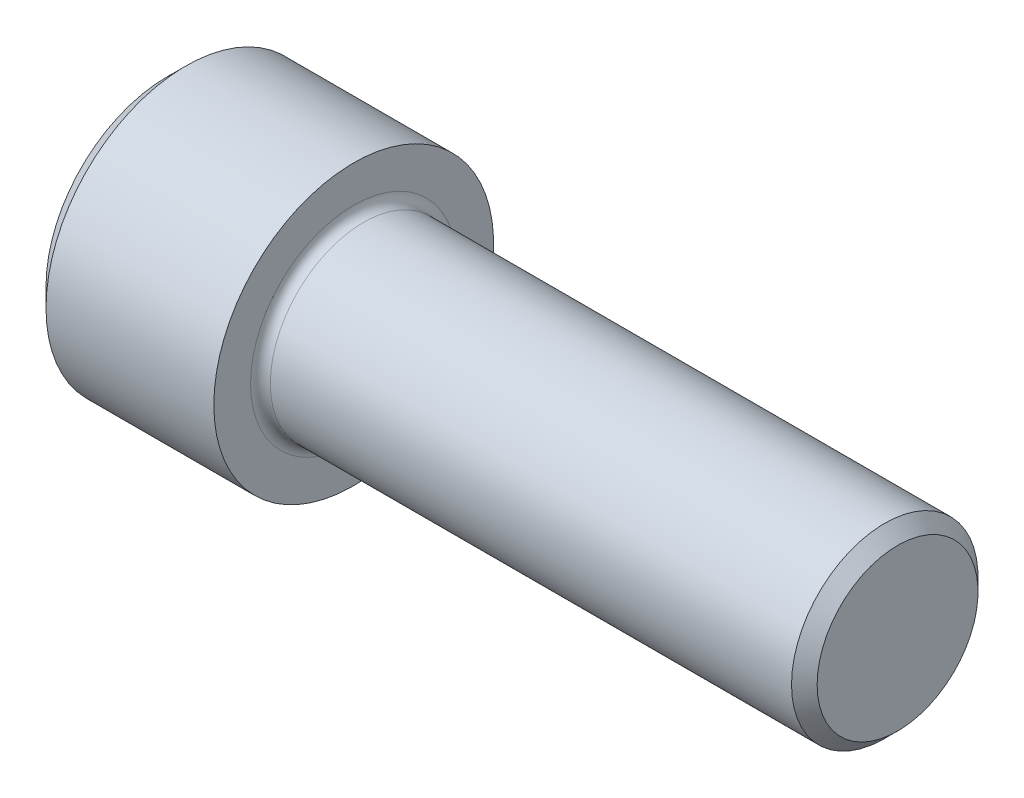
SolidWorks part; units mm, degrees
revolve "Base-Revolve" add sketch "BodySke"
sketch "BodySke" plane through (0, 0, 0) normal (0, 0, 1) x (1, 0, 0)
  line L0 (0, 0) -> (0, 15.6)
  line L1 (2.4, 18) -> (24, 18)
  line L2 (24, 18) -> (24, 12)
  line L3 (24, 12) -> (92.352, 12)
  line L4 (94, 10.352) -> (94, 0)
  line L5 (94, 0) -> (0, 0)
  line L6 (-31.75, 0) -> (127, 0) construction
  line L7 (0, 15.6) -> (2.4, 18)
  line L8 (94, 10.352) -> (92.352, 12)
  line L9 (0, -15.6) -> (2.4, -18) construction
  line L10 (94, -10.352) -> (92.352, -12) construction
  line L11 (27, 9.525) -> (27, 3.175) construction
  line L12 (44, 9.525) -> (44, 3.175) construction
  line L13 (44, 9.525) -> (44, 3.175) construction
  dimension "Diameter" = 24
  dimension "Head_ht" = 24
  dimension "Length" = 70
  dimension "Body_ch_ang" = 45
  dimension "Head_dia" = 36
  dimension "Head_ch_ang" = 45
  dimension "Minor_dia" = 20.704
  dimension "Advance" = 3
  dimension "Thread_nom" = 50
  dimension "Thread_length" = 50
  dimension "Head_ch_ht" = 2.4
cosmetic thread "ThreadCosmetic" [suppressed]
fillet "Fillet1" radius 1.27 1 edges at (24, 0, 12)
ref_plane "Plane1" through (0, 0, 0) normal (0, 0, 1) x (1, 0, 0)
ref_plane "Plane2" through (0, 0, 0) normal (0, 1, 0) x (1, 0, 0)
ref_plane "Plane3" through (0, 0, 0) normal (1, 0, 0) x (0, 0, -1)
other "Configuration Table"
sketch "Sketch2" plane through (0, 0, 0) normal (0, 0, 1) x (1, 0, 0)
  line L0 (0, 9.5) -> (12, 9.5)
  line L1 (12, 9.5) -> (17.4848, 0)
  line L2 (-31.75, 0) -> (127, 0) construction
  line L3 (17.4848, 0) -> (0, 0)
  line L4 (0, 0) -> (0, 9.5)
  line L5 (0, 15.6) -> (0, -15.6) construction
  line L6 (0, 0) -> (47.625, 0) construction
  line L7 (24, -18) -> (24, 18) construction
revolve "Hex-PreBroach" cut sketch "Sketch2" angle 360 about L6
sketch "Sketch3" plane through (0, 0, 0) normal (-1, 0, 0) x (0, 0.5, 0.866)
  line L0 (5.4848, 9.5) -> (-5.4848, 9.5)
  line L1 (-5.4848, 9.5) -> (-10.9697, 0)
  line L2 (5.4848, 9.5) -> (10.9697, 0)
  line L3 (5.4848, -9.5) -> (10.9697, 0)
  line L4 (5.4848, -9.5) -> (-5.4848, -9.5)
  line L5 (-5.4848, -9.5) -> (-10.9697, 0)
extrude "Hex" cut sketch "Sketch3" against normal blind 12
sketch "Sketch4" plane through (0, 0, 0) normal (-1, 0, 0) x (0, 0, 1)
  line L0 (0, 0) -> (10.1727, 0)
  line L1 (0, 0) -> (6.1484, 3.5498) construction
  line L2 (0, 0) -> (5.0863, 8.8098)
  line L3 (8.4417, 2.1022) -> (9.7612, 2.864)
  line L4 (6.0414, 6.2596) -> (7.3609, 7.0215)
  arc A0 (8.4417, 2.1022) -> (6.0414, 6.2596) centre (0, 0) ccw
  arc A1 (10.1727, 0) -> (9.7612, 2.864) centre (0, 0) ccw
  arc A2 (5.0863, 8.8098) -> (7.3609, 7.0215) centre (0, 0) cw
extrude "Spline" [suppressed] cut sketch "Sketch4" against normal blind 12.573
pattern_circular "CirPattern1" [suppressed] count 6 every 60
sketch "Sketch5" plane through (0, 0, 0) normal (0, 0, 1) x (1, 0, 0)
  line L0 (-31.75, 0) -> (127, 0) construction
  line L2 (0, 15.6) -> (0, -15.6) construction
  circle A0 centre (7.3, 0) radius 1.075
  dimension "Drilled_hole_dia" = 2.15
  dimension "Drilled_hole_loc" = 7.3
extrude "Hole" [suppressed] cut sketch "Sketch5" against normal through all and the other way through all
pattern_circular "Drilled-4" [suppressed] count 2 every 60
pattern_circular "Drilled-6" [suppressed] count 3 every 60
sketch "ThdSchSke" plane through (0, 0, 0) normal (0, 0, 1) x (1, 0, 0)
  line L0 (44, -10.352) -> (42.8461, -12)
  line L1 (44, -10.352) -> (45.1539, -12)
  line L2 (45.1539, -12) -> (45.1539, -15)
  line L3 (-3.175, 0) -> (5.1513, 0) construction
  line L5 (45.1539, -15) -> (42.8461, -15)
  line L6 (42.8461, -15) -> (42.8461, -12)
  line L7 (0, 15.6) -> (0, -15.6) construction
revolve "ThreadSchematic" [suppressed] cut sketch "ThdSchSke" angle 360 about L3
pattern_linear "ThdSchPat" [suppressed]
equation "\"D2@Sketch3\" = \"Hex_size@Sketch3\" / 2"
equation "\"D1@Sketch3\" = \"Hex_size@Sketch3\" / 2"
equation "\"D1@Sketch2\" = \"Hex_size@Sketch3\" / 2"
equation "\"D3@Sketch4\" = \"Spline_p_dim@Sketch4\" / 2"
equation "\"Thread_minor@ThreadCosmetic\"  =  \"Minor_dia@BodySke\""
equation "\"D2@CirPattern1\" = 360 / \"Num_teeth@CirPattern1\""
equation "\"Wall_thickness@Sketch2\" = \"Head_ht@BodySke\" - \"Key_eng@Hex\""
equation "\"Thread_length@ThreadCosmetic\" = ((sgn( (\"Length@BodySke\" - \"Advance@BodySke\" ) - \"Thread_nom@BodySke\" )-1)*( (\"Length@BodySke\" - \"Advance@BodySke\" ) - \"Thread_nom@BodySke\" ))/-2+ \"Thread_nom@BodySke\""
equation "\"Thread_minor@ThdSchSke\" = \"Minor_dia@BodySke\""
equation "\"Diameter@ThdSchSke\" = \"Diameter@BodySke\""
equation "\"Overcut@ThdSchSke\" = \"Diameter@BodySke\" * 1.25"
equation "\"Start@ThdSchSke\" = \"Head_ht@BodySke\" + \"Length@BodySke\" - \"Thread_length@ThreadCosmetic\"  '---Non-countersunk---"
equation "\"Num_threads@ThdSchPat\" = int( \"Thread_length@ThreadCosmetic\" / \"Advance@BodySke\" + 0.999 )  + 1"
equation "\"Advance@ThdSchPat\" = \"Thread_length@ThreadCosmetic\" /  (\"Num_threads@ThdSchPat\" - 1) 'relax it"
equation "\"Num_threads@ThdSchPat\" = \"Num_threads@ThdSchPat\" - sgn( \"Num_threads@ThdSchPat\" - 1) '---chamfered tips only---"
